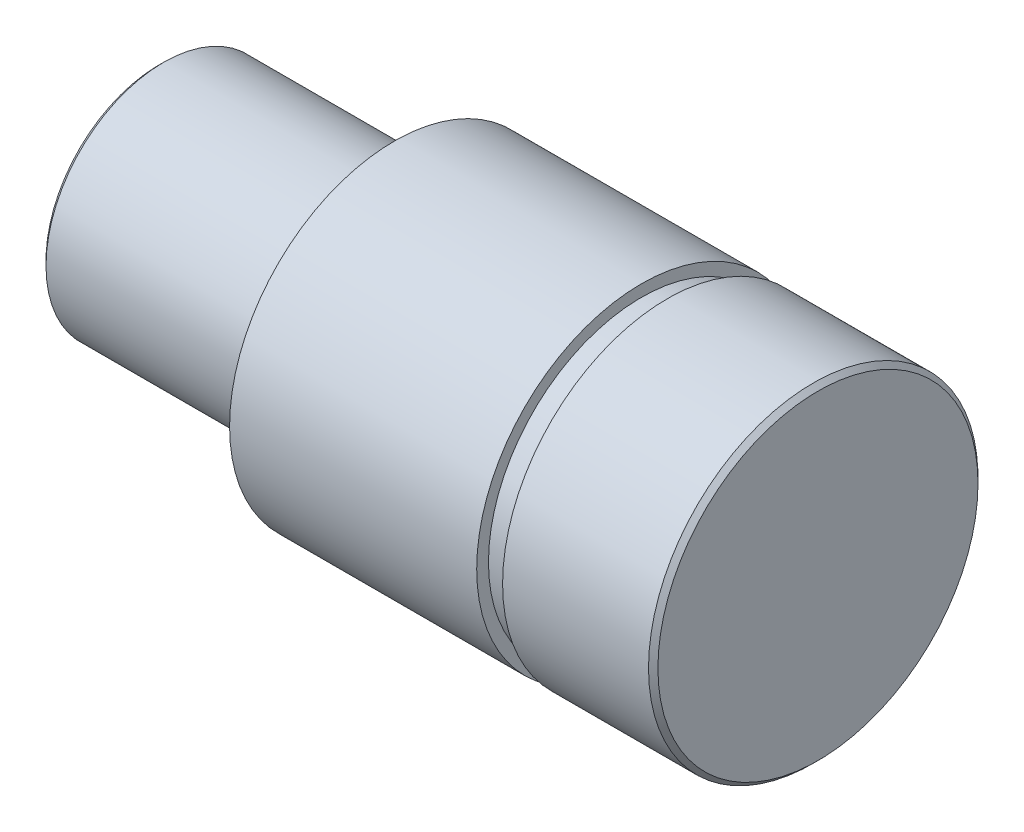
from build123d import *

# Parameters (mm, degrees)
CHAMFER1_SIZE = 0.2
CHAMFER2_SIZE = 0.2
SKETCH4_W     = 1.1
SKETCH4_H     = 2.393770958


with BuildPart() as part:
    # Sketch1 → Revolve1 (revolve)
    with BuildSketch(Plane.XY, mode=Mode.PRIVATE) as revolve1_sk:
        Polygon((0, 0), (0, 5), (10, 5), (10, 7), (28, 7), (28, 0), align=None)
    revolve(revolve1_sk.sketch.rotate(Axis((0, 0, 0), (1, 0, 0)), 90), axis=Axis((0, 0, 0), (1, 0, 0)))

    # Chamfer1
    chamfer1_edges = [part.edges().sort_by_distance(p)[0] for p in [
        (0, 0, -5),
    ]]
    chamfer(chamfer1_edges, length=CHAMFER1_SIZE)

    # Chamfer2
    chamfer2_edges = [part.edges().sort_by_distance(p)[0] for p in [
        (28, 0, -7),
    ]]
    chamfer(chamfer2_edges, length=CHAMFER2_SIZE)

    # Sketch4 → Cut-Revolve1 (revolve, cut)
    with BuildSketch(Plane(origin=(0, 0, 0), x_dir=(1, 0, 0), z_dir=(0, 1, 0)), mode=Mode.PRIVATE) as cut_revolve1_sk:
        with Locations((21.05, 7.696885479)):
            Rectangle(SKETCH4_W, SKETCH4_H)
    revolve(cut_revolve1_sk.sketch.rotate(Axis((0, 0, 0), (1, 0, 0)), 180), axis=Axis((0, 0, 0), (1, 0, 0)), mode=Mode.SUBTRACT)


solid = part.part
